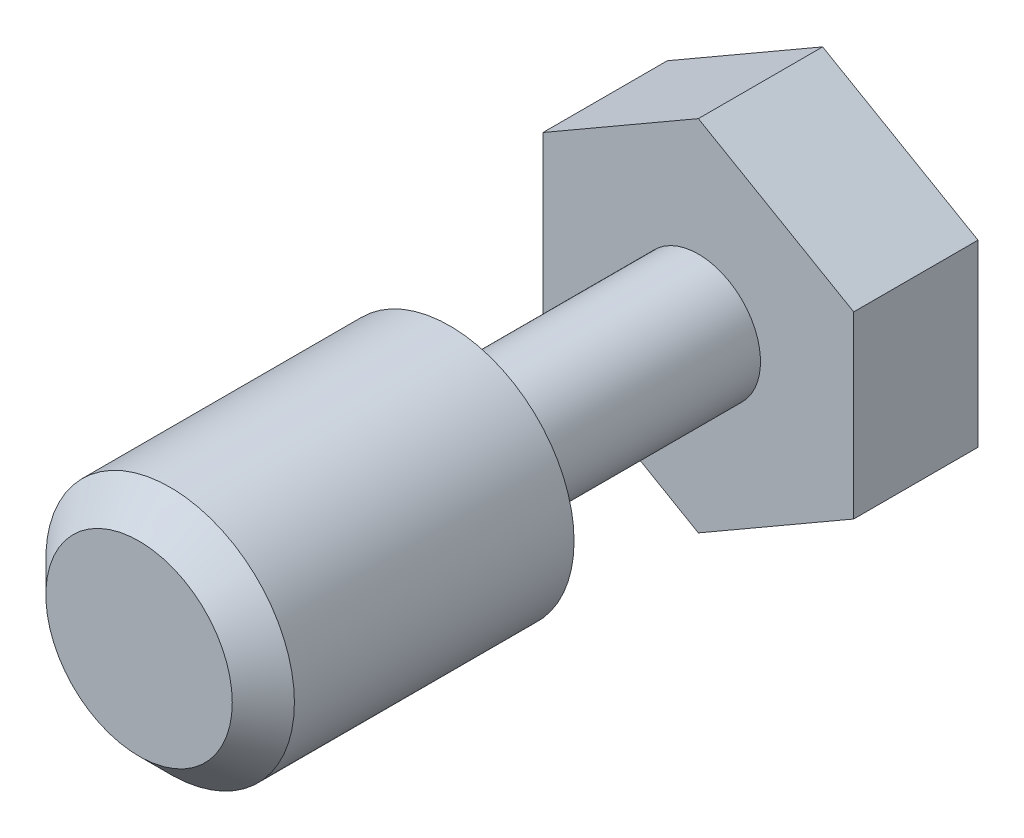
SolidWorks part; units mm, degrees
ref_plane "Front Plane" through (0, 0, 0) normal (0, 0, 1) x (1, 0, 0)
ref_plane "Top Plane" through (0, 0, 0) normal (0, 1, 0) x (1, 0, 0)
ref_plane "Right Plane" through (0, 0, 0) normal (1, 0, 0) x (0, 0, -1)
other "Configuration Table"
sketch "Sketch1" plane through (0, 0, 0) normal (0, 0, 1) x (1, 0, 0)
  circle A0 centre (0, 0) radius 2
  dimension "D1" = 4
extrude "Boss-Extrude1" add sketch "Sketch1" along normal blind 5
cosmetic thread "Cosmetic Thread1" parameters "D2"=3.8
sketch "Sketch2" plane through (0, 0, 0) normal (0, 0, -1) x (-1, 0, 0)
  circle A0 centre (0, 0) radius 1
  dimension "D1" = 2
extrude "Boss-Extrude2" add sketch "Sketch2" along normal blind 4
sketch "Sketch3" plane through (0, 0, -4) normal (0, 0, -1) x (-1, 0, 0)
  line L1 (0, 2.8868) -> (-2.5, 1.4434)
  line L2 (-2.5, 1.4434) -> (-2.5, -1.4434)
  line L3 (-2.5, -1.4434) -> (0, -2.8868)
  line L4 (0, -2.8868) -> (2.5, -1.4434)
  line L5 (2.5, -1.4434) -> (2.5, 1.4434)
  line L6 (2.5, 1.4434) -> (0, 2.8868)
  circle A0 centre (0, 0) radius 2.5 construction
  dimension "D1" = 5
extrude "Boss-Extrude3" add sketch "Sketch3" along normal blind 2
chamfer "Chamfer1" distance 0.5 angle 45 1 edges at (2, 0, 5)
